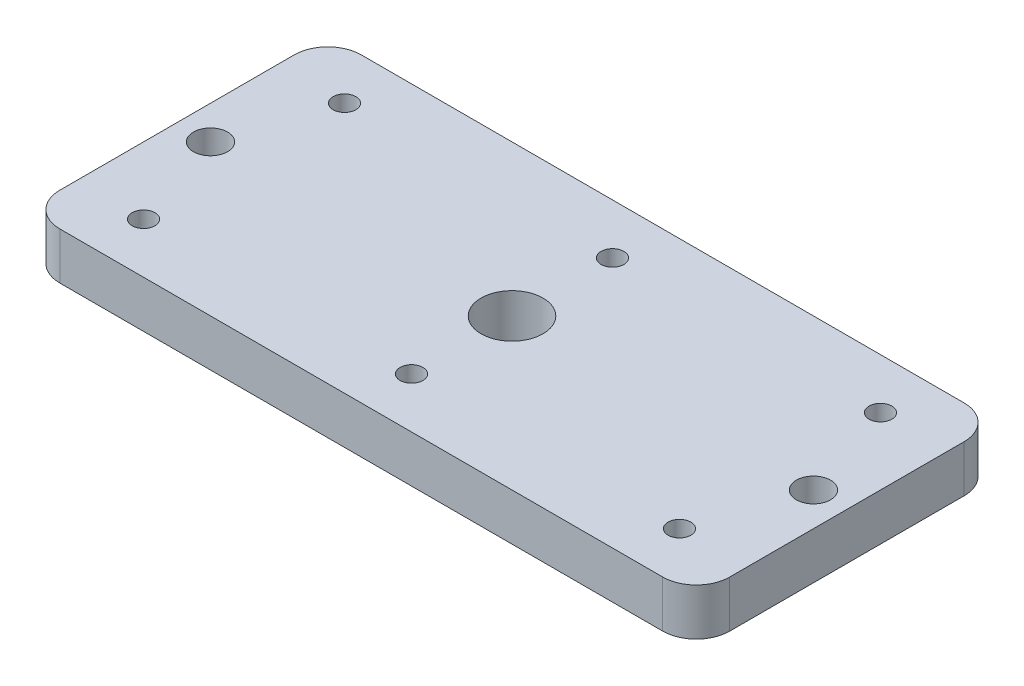
SolidWorks part; units mm, degrees
material "普通碳钢"
ref_plane "Front Plane" through (0, 0, 0) normal (0, 0, 1) x (1, 0, 0)
ref_plane "Top Plane" through (0, 0, 0) normal (0, 1, 0) x (1, 0, 0)
ref_plane "Right Plane" through (0, 0, 0) normal (1, 0, 0) x (0, 0, -1)
sketch "Sketch1" plane through (0, 0, 0) normal (0, 1, 0) x (1, 0, 0)
  line L1 (0, 0) -> (200, 0)
  line L2 (0, 0) -> (0, 90)
  line L3 (0, 90) -> (200, 90)
  line L4 (200, 0) -> (200, 90)
  dimension "D1" = 200
  dimension "D2" = 90
extrude "Boss-Extrude1" add sketch "Sketch1" along normal blind 14
hole_wizard "Socket Cap Screw Hole1" positions "Sketch2" profile "Sketch3" counterbore size "M8" standard "GB"
sketch "Sketch2" plane through (0, 14, 0) normal (0, 1, 0) x (1, 0, 0)
  line L0 (15, 85) -> (215, 85) construction
  line L1 (215, 85) -> (215, 15) construction
  line L2 (215, 15) -> (15, 15) construction
  line L3 (15, 15) -> (15, 85) construction
  line L5 (15, 50) -> (0, 50) construction
  line L6 (0, 100) -> (0, 0) construction
  line L8 (115, 15) -> (115, 0) construction
  line L9 (0, 0) -> (230, 0) construction
  point P0 (15, 85)
  point P2 (15, 15)
  point P4 (215, 15)
  point P6 (215, 85)
  dimension "D1" = 70
  dimension "D2" = 200
sketch "Sketch3" plane through (15, 14, -85) normal (1, 0, 0) x (0, 0, 1)
  line L0 (0, 0) -> (0, 14)
  line L1 (0, 14) -> (4.5, 14)
  line L3 (4.5, 14) -> (4.5, 9)
  line L4 (4.5, 9) -> (7.5, 9)
  line L5 (7.5, 9) -> (7.5, 0)
  line L7 (7.5, 0) -> (0, 0)
  line L11 (0, -6.35) -> (0, 107.95) construction
  dimension "通孔孔直径" = 9
  dimension "通孔孔深度" = 14
  dimension "柱形沉头孔直径" = 15
  dimension "柱形沉头孔深度" = 9
hole_wizard "M12 Tapped Hole1" positions "Sketch4" profile "Sketch5" tap size "M12" standard "GB"
sketch "Sketch4" plane through (0, 14, 0) normal (0, 1, 0) x (1, 0, 0)
  line L0 (0, 45) -> (10, 45) construction
  line L1 (0, 90) -> (0, 0) construction
  line L2 (10, 45) -> (190, 45) construction
  line L4 (100, 45) -> (100, 0) construction
  line L5 (0, 0) -> (200, 0) construction
  point P0 (10, 45)
  point P2 (190, 45)
  dimension "D1" = 180
sketch "Sketch5" plane through (10, 14, -45) normal (1, 0, 0) x (0, 0, 1)
  line L0 (0, 0) -> (0, 32.3144)
  line L1 (0, 32.3144) -> (5.1, 29.25)
  line L2 (5.1, 29.25) -> (5.1, 0)
  line L5 (5.1, 0) -> (0, 0)
  line L10 (0, 32.3144) -> (-5.1, 29.25) construction
  line L11 (0, -6.35) -> (0, 107.95) construction
  dimension "螺纹孔钻头直径" = 10.2
  dimension "螺纹孔钻头深度" = 29.25
  dimension "导头角度" = 118
cosmetic thread "Hole Thread2"
cosmetic thread "Hole Thread3"
fillet "Fillet1" radius 10 4 edges at (200, 7, -90) (200, 7, 0) (0, 7, -90) (0, 7, 0)
hole_wizard "M20x1.5 Tapped Hole1" positions "Sketch6" profile "Sketch7" tap size "M20x1.5" standard "GB" end condition through all
sketch "Sketch6" plane through (0, 14, 0) normal (0, 1, 0) x (1, 0, 0)
  line L0 (100, 0) -> (100, 45) construction
  line L1 (10, 0) -> (190, 0) construction
  line L2 (100, 45) -> (200, 45) construction
  line L3 (200, 10) -> (200, 80) construction
  point P0 (100, 45)
sketch "Sketch7" plane through (100, 14, -45) normal (1, 0, 0) x (0, 0, 1)
  line L0 (0, 0) -> (0, 14)
  line L1 (0, 14) -> (9.25, 14)
  line L2 (9.25, 14) -> (9.25, 0)
  line L5 (9.25, 0) -> (0, 0)
  line L11 (0, -6.35) -> (0, 107.95) construction
  dimension "通孔螺纹孔钻头直径" = 18.5
  dimension "通孔螺纹孔钻头深度" = 14
cosmetic thread "Hole Thread1" parameters "D2"=20
hole_wizard "M8 Tapped Hole1" positions "Sketch8" profile "Sketch9" tap size "M8" standard "GB" end condition through all
sketch "Sketch8" plane through (0, 14, 0) normal (0, 1, 0) x (1, 0, 0)
  line L0 (20, 75) -> (100, 75) construction
  line L1 (100, 75) -> (180, 75) construction
  line L2 (180, 75) -> (180, 15) construction
  line L3 (180, 15) -> (100, 15) construction
  line L4 (100, 15) -> (20, 15) construction
  line L5 (20, 15) -> (20, 75) construction
  line L7 (20, 45) -> (0, 45) construction
  line L8 (0, 80) -> (0, 10) construction
  line L10 (100, 15) -> (100, 0) construction
  line L11 (10, 0) -> (190, 0) construction
  line L13 (100, 15) -> (100, 75) construction
  point P0 (20, 75)
  point P2 (100, 75)
  point P4 (180, 75)
  point P6 (180, 15)
  point P8 (100, 15)
  point P10 (20, 15)
  dimension "D1" = 60
  dimension "D2" = 80
sketch "Sketch9" plane through (20, 14, -75) normal (1, 0, 0) x (0, 0, 1)
  line L0 (0, 0) -> (0, 14)
  line L1 (0, 14) -> (3.4, 14)
  line L2 (3.4, 14) -> (3.4, 0)
  line L5 (3.4, 0) -> (0, 0)
  line L11 (0, -6.35) -> (0, 107.95) construction
  dimension "通孔螺纹孔钻头直径" = 6.8
  dimension "通孔螺纹孔钻头深度" = 14
cosmetic thread "Hole Thread4"
cosmetic thread "Hole Thread5"
cosmetic thread "Hole Thread6"
cosmetic thread "Hole Thread7"
cosmetic thread "Hole Thread8"
cosmetic thread "Hole Thread9"
